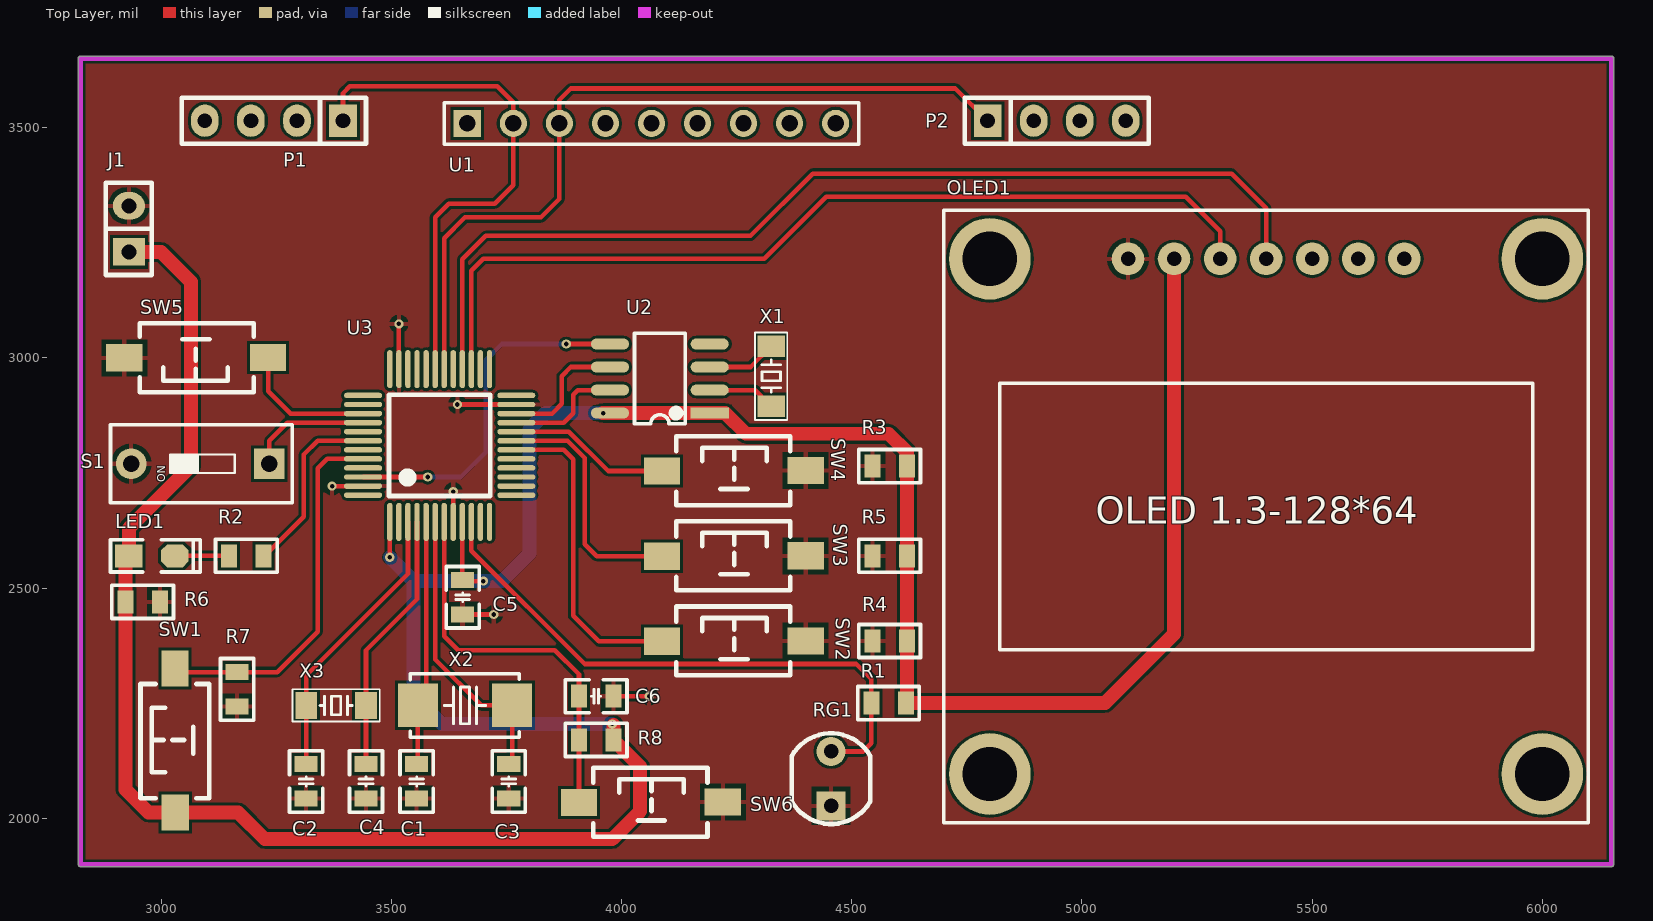
[diagram p0: Top Layer view]
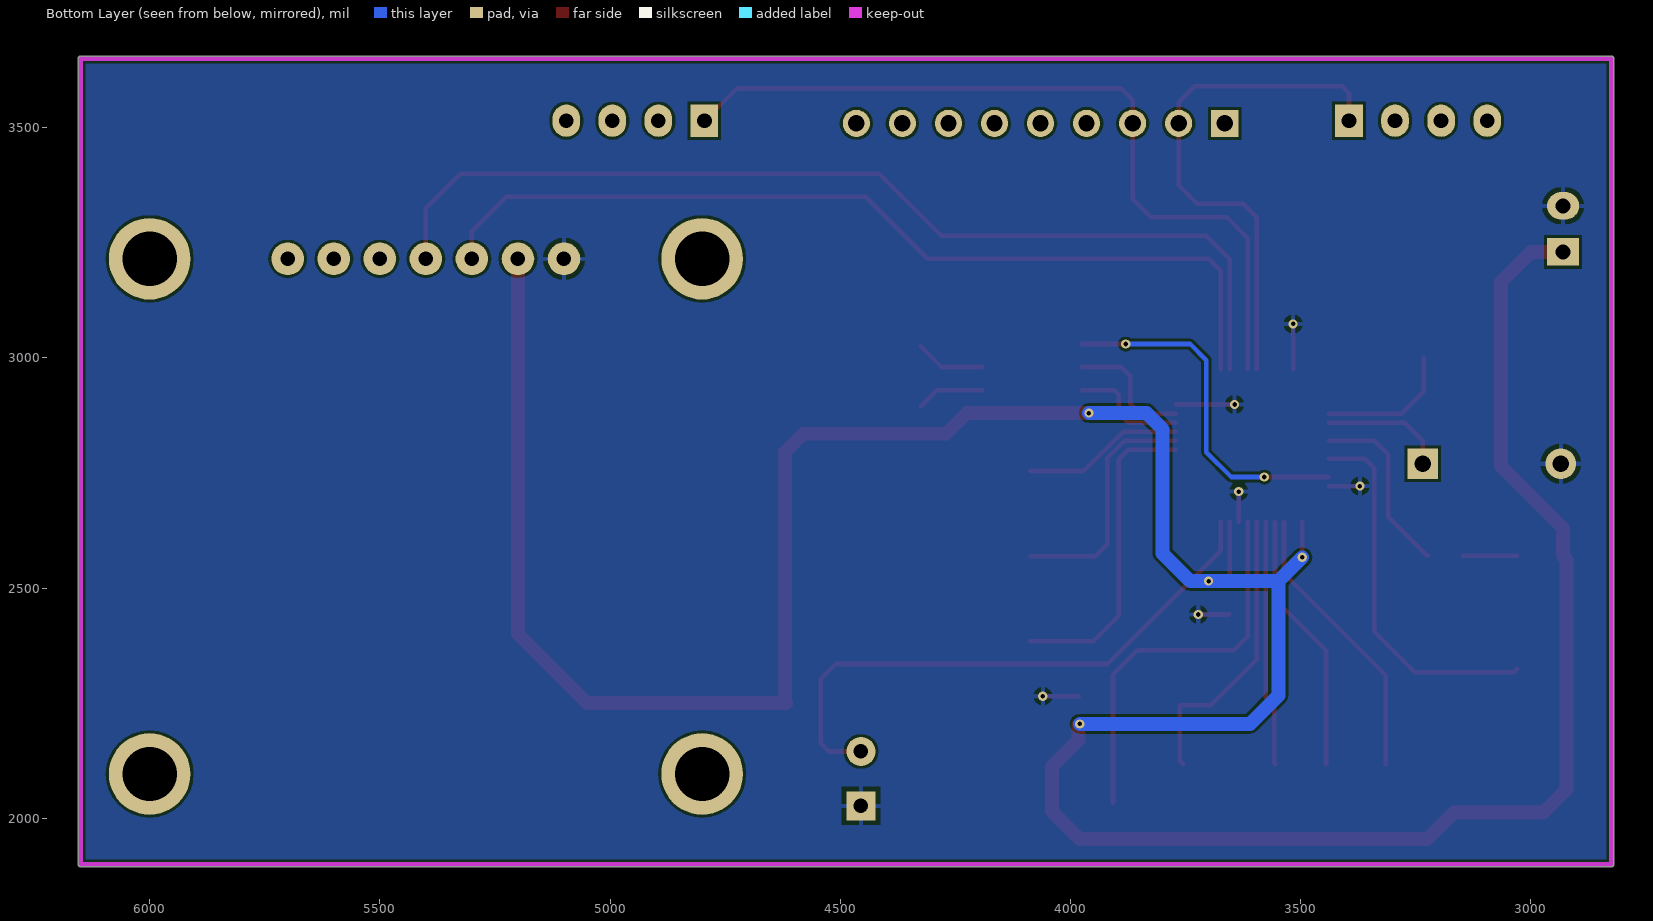
[diagram p1: Bottom Layer view, seen from below]
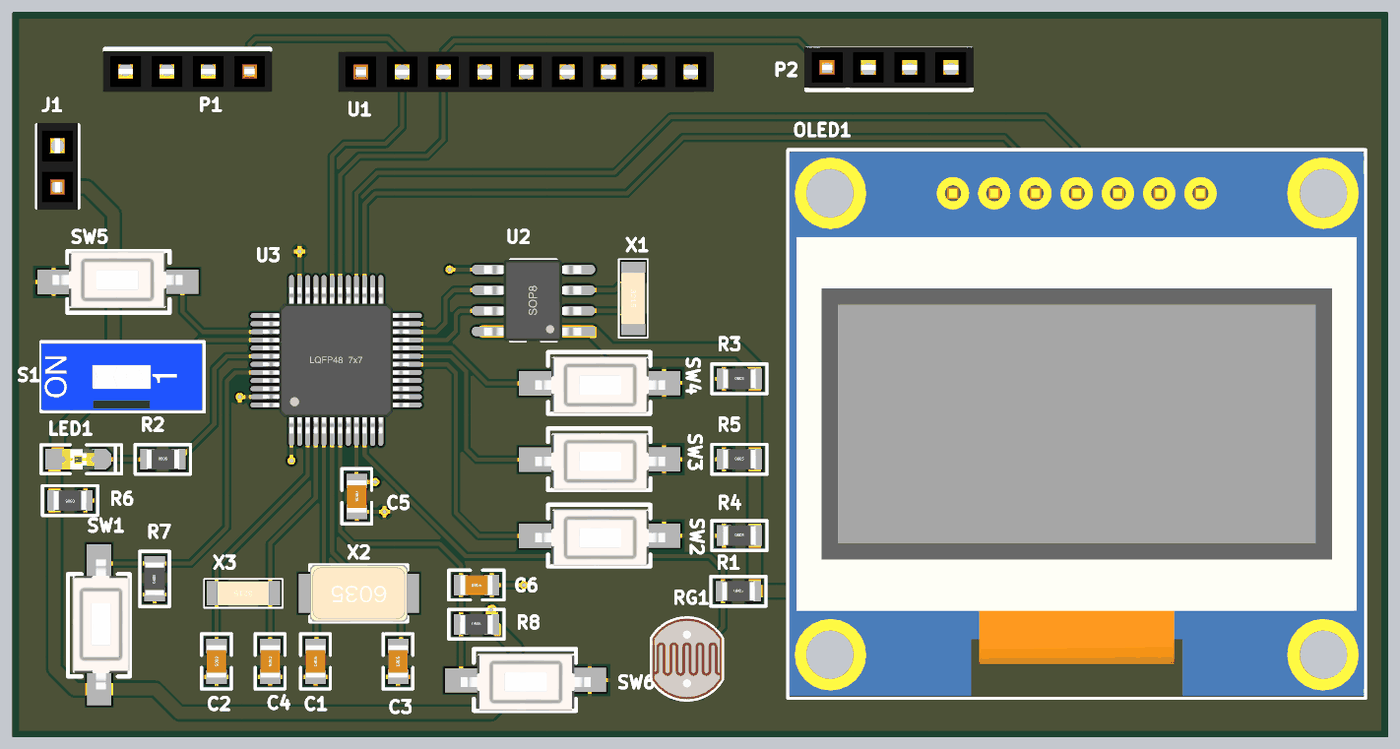
[diagram p2: 3D render of the assembled board from above, using the file's embedded part models]
# Altium PCB MISC80683.PcbDoc
Units mil, origin at the board's own origin, x right, y up, seen from the top; angles counter-clockwise.
Board outline 3335.03 x 1760.03 mil, 2 copper layers (Top Layer, Bottom Layer); 33 components, 25 nets, 138 pads, 12 vias.

## Layer stack, top to bottom (the 12.6 mil dielectric is the usual default, probably not edited)
Top Solder: solder mask 0.4, Solder Resist, Dk 3.5
Top Layer: signal copper 1.4
Dielectric 1: dielectric 12.6, FR-4, Dk 4.8
Bottom Layer: signal copper 1.4
Bottom Solder: solder mask 0.4, Solder Resist, Dk 3.5

## Board outline
2819.99,1900 ccw(c2825,1900) 2825,1894.98 6150,1894.98 ccw(c6150,1900) 6155.02,1900 6155.02,3650 ccw(c6150,3650) 6150,3655.01 2825,3655.01 ccw(c2825,3650) 2819.99,3650

## Design rules (kind name [scope] priority, off if disabled: settings)
Clearance [All] p1: gap=6
HoleSize [All] p1: absolutevalues=TRUE maxlimit=77777 minlimit=1 maxpercent=80.000 minpercent=20.000
MinimumSolderMaskSliver [All] p1: minsoldermaskwidth=0
PolygonConnect [All] p1: connectstyle=Relief reliefconductorwidth=10 reliefentries=4 polygonreliefangle="90 Angle" airgapwidth=10
RoutingVias [All] p1: holewidth=28 width=50 viastyle="Through Hole" minholewidth=28 minwidth=50 maxholewidth=28 maxwidth=50
SilkToSilkClearance [All] p1: silktosilkclearance=0
SilkToSolderMaskClearance [IsPad] p1: minsilkscreentomaskgap=0 clearancetoexposedcopper=TRUE
SolderMaskExpansion [All] p1: expansion=4
Width [All] p1: maxlimit=30 minlimit=10 preferedwidth=10
26 further rules are at their usual default settings.

## Components (designator, comment, footprint, x,y, rotation, side; value= is the part's Value field where it differs from the comment)
C1 "22pF" "C 0805_L" 3555,2080 r90 top
C2 "22pF" "C 0805_L" 3315,2080 r270 top
C3 "22pF" "C 0805_L" 3755,2080 r90 top
C4 "22pF" "C 0805_L" 3445,2080 r270 top
C5 "100nF" "C 0805_L" 3655,2480 r270 top
C6 "100nF" "C 0805_L" 3945,2265 r0 top
J1 "Female HDR1X2" Fe-HDR1X2/2.54-S 2930,3230 r90 top
LED1 "Red" "LED 0805G" 2980,2570 r0 top
OLED1 "OLED 1.3-12864_7pin" "OLED 1.3-12864_7pin" 5400,2655.55 r0 top
P1 "Header 4" Fe-HDR1X4/2.54-S 3395,3515 r270 top
P2 "Header 4" Fe-HDR1X4/2.54-S 4795,3515 r90 top
R1 "10K" "R 0805_L" 4580,2250 r0 top
R2 "10R" "R 0805_L" 3185,2570 r0 top
R3 "10K" "R 0805_L" 4582.4,2765 r0 top
R4 "10K" "R 0805_L" 4582.4,2385 r0 top
R5 "10K" "R 0805_L" 4582.4,2570 r0 top
R6 "10K" "R 0805_L" 2960,2470 r180 top
R7 "10K" "R 0805_L" 3165,2280 r90 top
R8 "10K" "R 0805_L" 3945,2170 r0 top
RG1 "10K" RG5528 4455,2026.89 r90 top
S1 "KCD1-101" "CSW DIP-1P" 3085,2770 r90 top
SW1 "3x6x5" "TSW SMD-3*6*2.5" 3030,2170 r90 top
SW2 "3x6x5" "TSW SMD-3*6*2.5" 4245,2385 r0 top
SW3 "3x6x5" "TSW SMD-3*6*2.5" 4245,2570 r0 top
SW4 "3x6x5" "TSW SMD-3*6*2.5" 4245,2755 r0 top
SW5 "3x6x5" "TSW SMD-3*6*2.5" 3075,3000 r180 top
SW6 "3x6x5" "TSW SMD-3*6*2.5" 4065,2035 r0 top
U1 "COMPIM" Fe-HDR1X9/2.54-S 3665,3509.21 r90 top
U2 "DS1302" SOP8 4191.54,2880 r180 top
U3 "STM32F103C8T6" "LQFP48 7X7" 3605,2810 r0 top
X1 "32.768K" "OSC 3215-2P" 4325,2960 r270 top
X2 "8MHz" "OSC 6035-2P" 3660,2245 r180 top
X3 "32.768K" "OSC 3215-2P" 3380,2245 r180 top

## Footprints (in the part's own frame and the unit in brackets; to place one, negate y for a bottom-side part, rotate by r counter-clockwise, add the part's x,y. Pads: shape width x height; smd on the part's side, far side on the other; paste and mask are expansions set on the pad)
"C 0805_L" [mil] "无极性贴片电容"
  rect 35x50 smd: 1(-37.4,0) 2(37.4,0)
  silkscreen extent -67,-36 67,36, body extent -39,-24 39,24, height 20
"CSW DIP-1P" [mm] "4.1*9.9*7mm"
  rect 1.7x1.7 hole 0.9: 1(0,-3.81)
  round 1.7 hole 0.9: 2(0,3.81)
  silkscreen extent -2.16,-5.08 2.16,4.95, body extent -2.05,-4.95 2.05,4.95, height 6.65
Fe-HDR1X2/2.54-S [mil] "Connector; Header; 2x2 Position"
  rect 60x70 hole 32: 1(0,0)
  oval 60x70 hole 32: 2(100,0)
  silkscreen extent -50,-50 150,50, body extent -55,-48 155,50, height 335
Fe-HDR1X4/2.54-S [mil]
  rect 70x60 hole 32: 1(0,0)
  oval 70x60 hole 32: 2(0,-100) 3(0,-200) 4(0,-300)
  silkscreen extent -50,-350 50,50, body extent -44,-355 54,55, height 335
Fe-HDR1X9/2.54-S [mm]
  rect 1.5x1.5 hole 0.9: 1(0,0)
  round 1.5 hole 0.9: 2(0,-2.54) 3(0,-5.08) 4(0,-7.62) 5(0,-10.16) 6(0,-12.7) 7(0,-15.24) 8(0,-17.78) 9(0,-20.32)
  silkscreen extent -1.14,-21.59 1.14,1.27, body extent -1.25,-21.72 1.25,1.4, height 3.2
"LED 0805G" [mil] "绿色0805LED"
  rect 60x50 smd: 1(-50,0)
  oct 60x50 smd: 2(50,0)
  silkscreen extent -90,-35 105,35, body extent -39,-25 39,25, height 32
"LQFP48 7X7" [mm]
  oval 0.3x2.1 smd: 1(-2.75,-4.227) 2(-2.25,-4.227) 3(-1.75,-4.227) 4(-1.25,-4.227) 5(-0.75,-4.227) 6(-0.25,-4.227) 7(0.25,-4.227) 8(0.75,-4.227) 9(1.25,-4.227) 10(1.75,-4.227) 11(2.25,-4.227) 12(2.75,-4.227) 25(2.75,4.202) 26(2.25,4.202) 27(1.75,4.202) 28(1.25,4.202) 29(0.75,4.202) 30(0.25,4.202) 31(-0.25,4.202) 32(-0.75,4.202) 33(-1.25,4.202) 34(-1.75,4.202) 35(-2.25,4.202) 36(-2.75,4.202)
  oval 2.1x0.3 smd: 13(4.227,-2.75) 14(4.227,-2.25) 15(4.227,-1.75) 16(4.227,-1.25) 17(4.227,-0.75) 18(4.227,-0.25) 19(4.227,0.25) 20(4.227,0.75) 21(4.227,1.25) 22(4.227,1.75) 23(4.227,2.25) 24(4.227,2.75) 37(-4.227,2.75) 38(-4.227,2.25) 39(-4.227,1.75) 40(-4.227,1.25) 41(-4.227,0.75) 42(-4.227,0.25) 43(-4.227,-0.25) 44(-4.227,-0.75) 45(-4.227,-1.25) 46(-4.227,-1.75) 47(-4.227,-2.25) 48(-4.227,-2.75)
  silkscreen extent -2.79,-2.79 2.79,2.79, body extent -4.51,-4.5 4.5,4.5, height 1.45
"OLED 1.3-12864_7pin" [mm] "长：35.4mm，宽：33.5mm，"
  round 4.5 hole 3: 0(-15.24,-14.21) 0(-15.24,14.21) 0(15.24,-14.21) 0(15.24,14.21)
  round 1.8 hole 0.8: 1(-7.62,14.21) 2(-5.08,14.21) 3(-2.54,14.21) 4(0,14.21) 5(2.54,14.21) 6(5.08,14.21) 7(7.62,14.21)
  silkscreen extent -17.78,-16.89 17.78,16.89, body extent -17.7,-16.75 17.7,16.75, height 5.5
"OSC 3215-2P" [mm] "3.2*1.5*0.6mm(长宽高)"
  rect 1.2x1.5 smd: 1(-1.65,0) 2(1.65,0)
  silkscreen extent -2.41,-0.89 2.41,0.89, body extent -1.6,-0.75 1.6,0.75, height 0.61
"OSC 6035-2P" [mm] "6mm*3.5mm*1mm(长*宽*高)"
  rect 2.2x2.4 smd: 1(-2.6,0) 2(2.6,0)
  silkscreen extent -3,-1.75 3.02,1.75, body extent -3,-1.75 3,1.75, height 1.06
"R 0805_L" [mil] "1/8W贴片电阻"
  rect 35x50 smd: 1(-37.4,0) 2(37.4,0)
  silkscreen extent -67,-36 67,36, body extent -39,-25 39,25, height 20
RG5528 [mm]
  rect 1.6x1.6 hole 0.8: 1(0,0)
  round 1.6 hole 0.8: 2(3,0)
  silkscreen extent -1,-2.16 4,2.16, body extent -1,-2.16 4,2.14, height 1.9
SOP8 [mm]
  rect 2.1x0.6 smd: 1(0,0)
  oval 2.1x0.6 smd: 2(0,-1.27) 3(0,-2.54) 4(0,-3.81) 5(5.5,-3.81) 6(5.5,-2.54) 7(5.5,-1.27) 8(5.5,0)
  silkscreen extent 1.35,-4.41 4.15,0.6, body extent -0.21,-4.4 5.8,0.6, height 1.9
"TSW SMD-3*6*2.5" [mm] "3*6*2.5mm"
  rect 2x1.5 smd: 1(-3.996,-0.02) 2(3.937,0)
  silkscreen extent -3.21,-1.9 3.09,1.9, body extent -4,-1.88 4,1.62, height 2.59

## Part data
C1 C2 C3 C4 C5 C6: library part C, "Chip capacitor"
LED1: library part LED-SMD, "Chip LED"
OLED1: "12864 dot-matrix display"
P1 P2: "Header, 4-Pin"
R1 R2 R3 R4 R5 R6 R7 R8: library part R, "Chip resistor"
RG1: library part RG, "Photoresistor"
S1: "1-circuit SPST boat-type switch"
SW1 SW2 SW3 SW4 SW5 SW6: library part "TSW 3x6", "3x6 tactile switch"
U2: "Trickle Charge Timekeeping Chip"
X1 X2 X3: library part XTAL-2P, "2-pin passive crystal"

## Via types
v1: diameter 20, hole 10, Top Layer to Bottom Layer, 12 vias

## Nets (pads, with @x,y where several pads share a name; then routed paths per layer and width w, separated by ;. In a path a pad name is that pad's centre, name@x,y a point inside that pad or via, vN(x,y) a via of type N, cw(c..) or ccw(c..) an arc to the next point about the centre after c; other vN are vias at no path point)
+3.3V: C5.1 J1.1 LED1.1 OLED1.2 R1.2 R3.2 R4.2 R5.2 R6.2 R8.2 SW1.1 U2.1 U2.8 U3.1 U3.9 | length 7171.5
  Top Layer w10: v1(3496.73,2566.73) U3.1 ; U3.9 3654.21,2518.19 C5.1 3657.4,2515 v1(3700,2515)
  Top Layer w30: J1.1 3000,3230 3065,3165 3065,2765 2930,2630 LED1.1 2922.6,2562.6 R6.2 2922.6,2062.4 2972.31,2012.69 SW1.1 3167.31,2012.69 3225,1955 3980,1955 4040,2015 4040,2112.4 R8.2 v1@3982.4,2202.6 ; v1(3960,2880) U2.8 U2.1 4225,2880 4270,2835 4580,2835 4619.8,2795.2 R3.2 R5.2 R4.2 4619.8,2252.4 R1.2 5050,2250 5200,2400 OLED1.2
  Bottom Layer w30: v1(3496.73,2566.73) 3548.46,2515 ; v1(3960,2880) 3835,2880 3800,2845 3800,2575 3740,2515 v1(3700,2515) 3548.46,2515 ; v1(3980,2205) 3610,2205 3548.46,2266.54 3548.46,2515
GND: C1.1 C2.2 C3.1 C4.2 C5.2 C6.2 J1.2 OLED1.1 R3.1 R4.1 R5.1 R6.1 R7.1 RG1.1 S1.2 SW2.2 SW3.2 SW4.2 SW5.2 SW6.2 U3.8 U3.23 U3.35 U3.47 | length 504.1
  Top Layer w10: v1(3371.42,2721.42) U3.47 ; U3.35 v1(3516.42,3073.58) ; U3.8 v1(3634.53,2709.53) ; v1(3643.58,2898.58) U3.23 ; C5.2 v1(3722.4,2442.6) ; C6.2 v1(4060,2265)
IO: U2.6 U3.22 | length 280.6
  Top Layer w10: U3.22 3848.9,2878.9 3870,2900 3870,2960 3890,2980 U2.6
KEY1: SW2.1 U3.18 | length 687.7
  Top Layer w10: U3.18 3874.84,2800.16 3895,2780 3895,2440 3950.79,2384.21 SW2.1
KEY2: SW3.1 U3.19 | length 529.8
  Top Layer w10: U3.19 3882.53,2819.84 3920,2782.37 3920,2595 3945.79,2569.21 SW3.1
KEY3: SW4.1 U3.20 | length 351.6
  Top Layer w10: U3.20 3885.47,2839.53 3970.79,2754.21 SW4.1
KEY4: SW5.1 U3.39 | length 299.6
  Top Layer w10: SW5.1 3232.31,2927.69 3281.1,2878.9 U3.39
LDR: R1.1 RG1.2 U3.10 | length 1281.3
  Top Layer w10: U3.10 3673.9,2581.1 3920,2335 4510,2335 4542.6,2302.4 R1.1 4542.6,2162.6 4525,2145 RG1.2
NetC1_2: C1.2 U3.5 X2.2 | length 534.7
  Top Layer w10: C1.2 3557.64,2120.04 X2.2 3575.47,2262.83 U3.5
NetC2_1: C2.1 U3.3 X3.2 | length 617.8
  Top Layer w10: C2.1 C2.1 X3.2 3315.04,2310.04 3536.1,2531.1 U3.3
NetC3_2: C3.2 U3.6 X2.1 | length 638
  Top Layer w10: U3.6 3595.16,2344.84 3695,2245 X2.1 3762.36,2124.76 C3.2
NetC4_1: C4.1 U3.4 X3.1 | length 572.1
  Top Layer w10: C4.1 C4.1 X3.1 3444.96,2364.96 3555.79,2475.79 U3.4
NetC6_1: C6.1 R8.1 SW6.1 U3.7 | length 853.7
  Top Layer w10: U3.7 3614.84,2395.16 3645,2365 3855,2365 3907.6,2312.4 C6.1 3907.69,2264.91 SW6.1
NetLED1_2: LED1.2 R2.1 | length 117.6
  Top Layer w10: LED1.2 R2.1
NetR7_2: R7.2 SW1.2 U3.44 | length 811.5
  Top Layer w10: SW1.2 3037.6,2317.4 R7.2 3252.4,2317.4 3340,2405 3340,2760 3360.47,2780.47 U3.44
NetU2_2: U2.2 X1.2 | length 147.9
  Top Layer w10: U2.2 4290.04,2930 X1.2
NetU2_3: U2.3 X1.1 | length 152.1
  Top Layer w10: U2.3 4280.04,2980 X1.1
PWM: R2.2 U3.42 | length 398.8
  Top Layer w10: R2.2 3225,2570 3310,2655 3310,2790 3339.84,2819.84 U3.42
R: S1.1 U3.40 | length 269.8
  Top Layer w10: S1.1 3235,2820 3274.21,2859.21 U3.40
RST: U2.5 U3.46 | length 774.8
  Top Layer w10: U3.46 v1(3578.9,2741.1) v1@3580,2740 ; v1(3880,3030) U2.5
  Bottom Layer w10: v1(3578.9,2741.1) 3651.1,2741.1 3705,2795 3705,2995 3740,3030 v1(3880,3030)
RX1: P1.1 U1.2 U3.31 | length 1159.2
  Top Layer w10: P1.1 3395,3575 3410,3590 3730,3590 3765,3555 U1.2 3765,3375 3725,3335 3625,3335 3595.16,3305.16 U3.31
SCL: OLED1.3 U3.27 | length 1997.4
  Top Layer w10: U3.27 3673.9,3188.9 3700,3215 4310,3215 4445,3350 5225,3350 5300,3275 OLED1.3
SCLK: U2.7 U3.21 | length 256.3
  Top Layer w10: U3.21 3874.21,2859.21 3895,2880 3895,2920 3905,2930 U2.7
SDA: OLED1.4 U3.28 | length 2202.6
  Top Layer w10: U3.28 3654.21,3214.21 3705,3265 4280,3265 4415,3400 5325,3400 5400,3325 OLED1.4
TX1: P2.1 U1.3 U3.30 | length 1754.2
  Top Layer w10: U3.30 3614.84,3259.84 3660,3305 3825,3305 3865,3345 U1.3 3865,3560 3890,3585 4725,3585 P2.1
pads on no net: OLED1.0 OLED1.5 OLED1.6 OLED1.7 P1.2 P1.3 P1.4 P2.2 P2.3 P2.4 U1.1 U1.4 U1.5 U1.6 U1.7 U1.8 U1.9 U2.4 U3.2 U3.11 U3.12 U3.13 U3.14 U3.15 U3.16 U3.17 U3.24 U3.25 U3.26 U3.29 U3.32 U3.33 U3.34 U3.36 U3.37 U3.38 U3.41 U3.43 U3.45 U3.48

## Polygon pours and split planes (outlines as drawn)
GND on Top Layer "D" (solid, remove dead copper, pour order 10): 2700,3785 6310,3785 6310,1790 6335,1765 6265,1835 2855,1835 2825,1835 2820,1830
GND on Bottom Layer "D" (solid, remove dead copper, pour order 12): 2680,3785 2715,3750 6105,3750 6445,3750 6215,3520 6215,1800 2815,1800 2750,1735

## Keep-outs
Keep-Out Layer:
  lines w10: 2825,1900 2825,3650 6150,3650 6150,1900 2825,1900